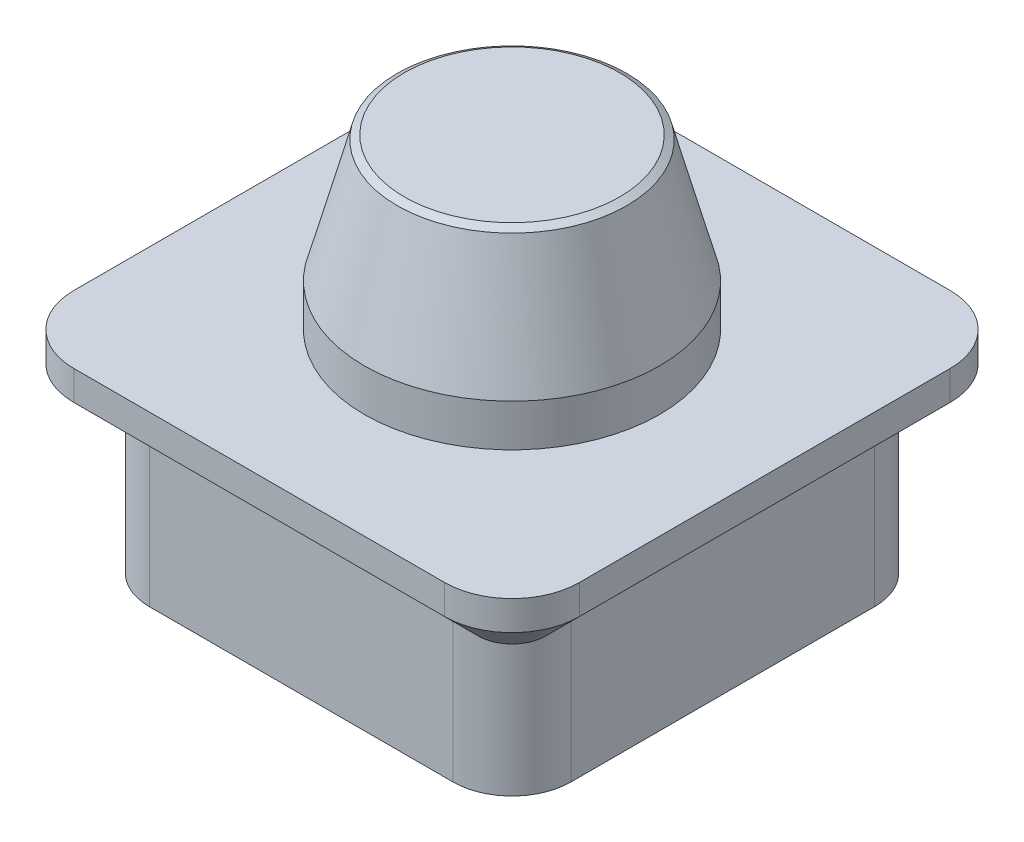
from build123d import *

# Parameters (mm, degrees)
CHAMFER1_SIZE       = 1
CHAMFER1_SIZE2      = 1.414213562
BOSS_EXTRUDE1_DEPTH = 15
BOSS_EXTRUDE2_DEPTH = 35
CHAMFER2_SIZE       = 8


with BuildPart() as part:
    # feature 17 (ProfileFeature) (+16 more in 12 files) Sketch1 → Revolve1 (revolve)
    with BuildSketch(Plane.XY, mode=Mode.PRIVATE) as revolve1_sk:
        Polygon((0, 0), (35, 0), (35, 10), (26.961524227, 40), (0, 40), align=None)
    revolve(revolve1_sk.sketch.rotate(Axis((0, 40, 0), (0, -1, 0)), 180), axis=Axis((0, 40, 0), (0, -1, 0)))

    # Chamfer1
    chamfer1_edges = [part.edges().sort_by_distance(p)[0] for p in [
        (26.961524227, 40, 0),
    ]]
    chamfer1_side = [part.faces().sort_by_distance(p)[0] for p in [
        (30.980762114, 25, 0),
    ]]
    chamfer(chamfer1_edges, length=CHAMFER1_SIZE, length2=CHAMFER1_SIZE2, reference=chamfer1_side[0])

    # 0:feat:20/0 feature 20/0 (ProfileFeature) (+11 more in 7 files) Sketch2 → Boss-Extrude1 (add)
    with BuildSketch(Plane.XZ):
        with BuildLine():
            Line((44, -60), (-44, -60))
            ThreePointArc((-44, -60), (-55.313708499, -55.313708499), (-60, -44))
            Line((-60, -44), (-60, 44))
            ThreePointArc((-60, 44), (-55.313708499, 55.313708499), (-44, 60))
            Line((-44, 60), (44, 60))
            ThreePointArc((44, 60), (55.313708499, 55.313708499), (60, 44))
            Line((60, 44), (60, -44))
            ThreePointArc((60, -44), (55.313708499, -55.313708499), (44, -60))
        make_face()
    extrude(amount=BOSS_EXTRUDE1_DEPTH)

    # 0:feat:20/1 feature 20/1 (ProfileFeature) (+2 more in 2 files) Sketch3 → Boss-Extrude2 (add)
    with BuildSketch(Plane.XZ.offset(15)):
        with BuildLine():
            Line((36, -50), (-36, -50))
            ThreePointArc((-36, -50), (-45.899494937, -45.899494937), (-50, -36))
            Line((-50, -36), (-50, 36))
            ThreePointArc((-50, 36), (-45.899494937, 45.899494937), (-36, 50))
            Line((-36, 50), (36, 50))
            ThreePointArc((36, 50), (45.899494937, 45.899494937), (50, 36))
            Line((50, 36), (50, -36))
            ThreePointArc((50, -36), (45.899494937, -45.899494937), (36, -50))
        make_face()
    extrude(amount=BOSS_EXTRUDE2_DEPTH)

    # Chamfer2
    chamfer2_edges = [part.edges().sort_by_distance(p)[0] for p in [
        (-55.313708499, -15, -55.313708499),
        (0, -15, -60),
        (55.313708499, -15, -55.313708499),
        (60, -15, 0),
        (55.313708499, -15, 55.313708499),
        (0, -15, 60),
        (-55.313708499, -15, 55.313708499),
        (-60, -15, 0),
    ]]
    chamfer(chamfer2_edges, length=CHAMFER2_SIZE)


solid = part.part
